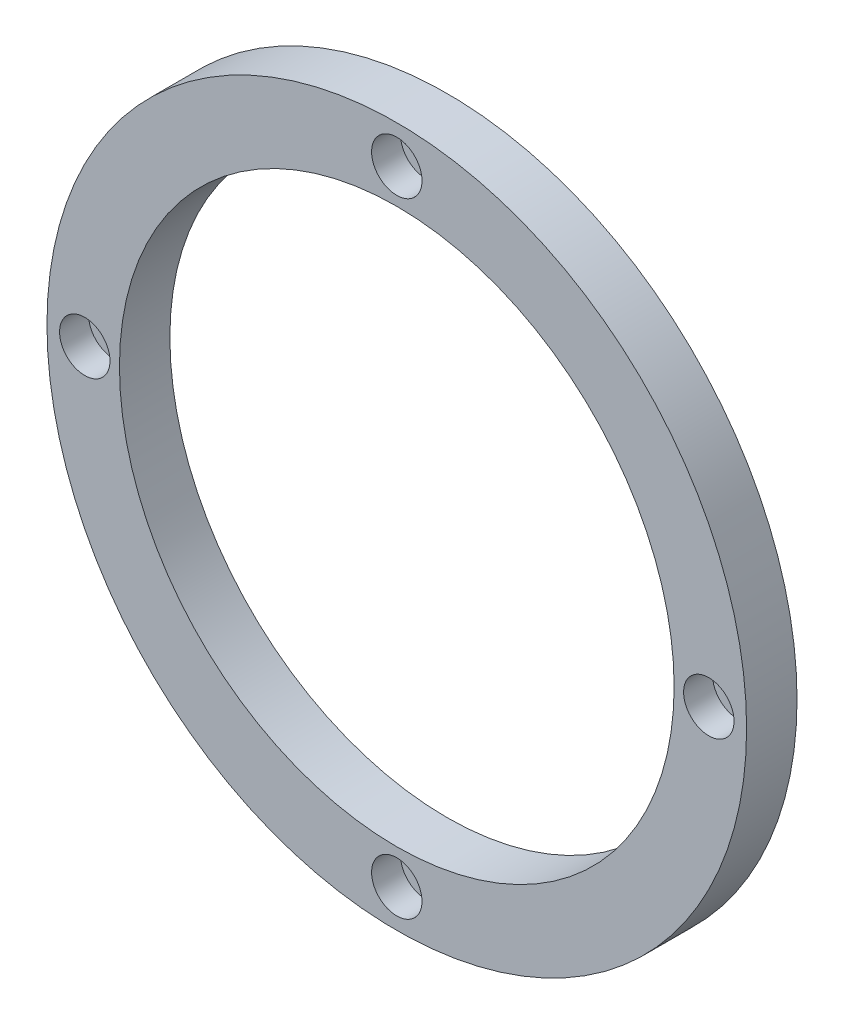
from build123d import *

# Parameters (mm, degrees)
SKETCH1_R           = 55.5
SKETCH1_R_2         = 44
BOSS_EXTRUDE1_DEPTH = 8
CIRPATTERN1_COUNT   = 4


with BuildPart() as part:
    # Sketch1 → Boss-Extrude1 (new body)
    with BuildSketch(Plane.XY):
        Circle(SKETCH1_R)
        Circle(SKETCH1_R_2, mode=Mode.SUBTRACT)
    extrude(amount=BOSS_EXTRUDE1_DEPTH)

    # Sketch5 → Hole size per socket head cap screw type 1 (revolve, cut)
    with BuildSketch(Plane(origin=(0, 49.5, 8), x_dir=(0, -1, 0), z_dir=(1, 0, 0))):
        Polygon((0, 0), (0, 18.351936393), (2.25, 17), (2.25, 4.6), (4, 4.6), (4, 0), align=None)
    hole_size_per_socket_head_cap_screw_type = revolve(axis=Axis((0, 49.5, 14.35), (0, 0, -1)), mode=Mode.SUBTRACT)

    # CirPattern1: Hole size per socket head cap screw type 1 ×4 about axis
    cirpattern1_axis = Axis((0, 0, 0), (0, 0, 1))
    for i in range(1, CIRPATTERN1_COUNT):
        add(hole_size_per_socket_head_cap_screw_type.rotate(cirpattern1_axis, i * 360 / CIRPATTERN1_COUNT), mode=Mode.SUBTRACT)


solid = part.part
